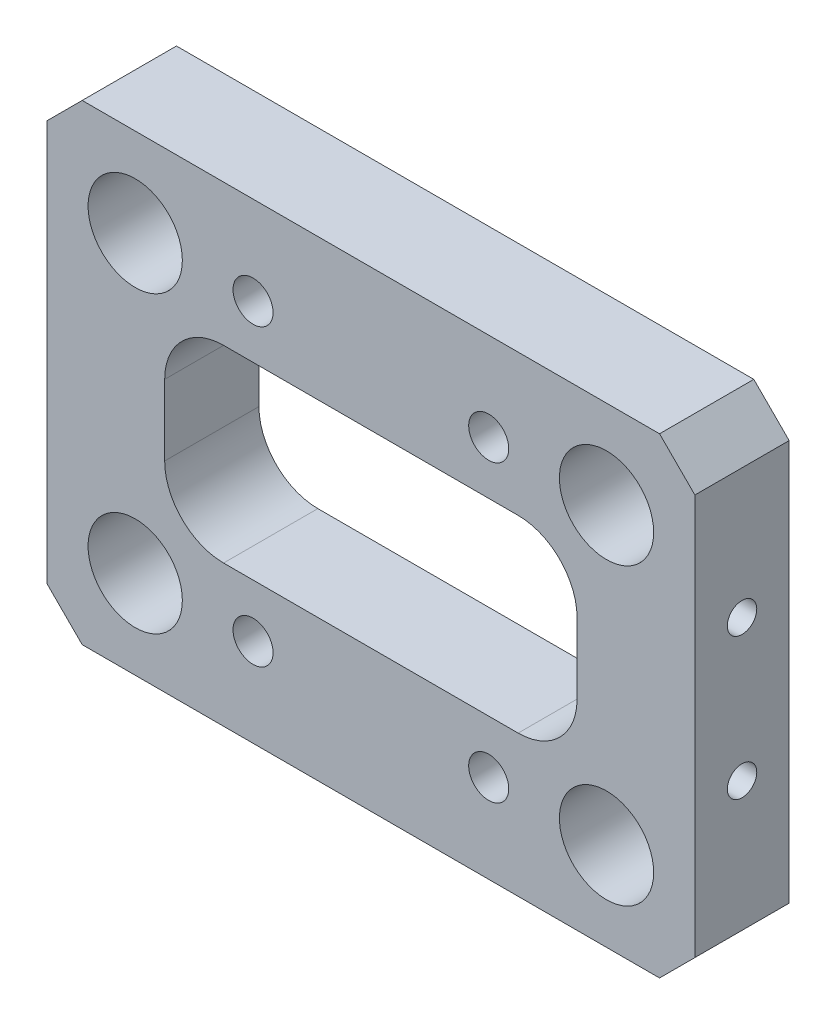
SolidWorks part; units mm, degrees
material "6061-T6 (SS)"
ref_plane "Front" through (0, 0, 0) normal (0, 0, 1) x (1, 0, 0)
ref_plane "Top" through (0, 0, 0) normal (0, 1, 0) x (1, 0, 0)
ref_plane "Right" through (0, 0, 0) normal (1, 0, 0) x (0, 0, -1)
ref_plane "基准面1" through (0, 0, 4) normal (0, 0, 1) x (1, 0, 0)
sketch "草图1" plane through (0, 0, 4) normal (0, 0, 1) x (1, 0, 0)
  line L0 (-27.5, 20) -> (-27.5, -20)
  line L1 (-27.5, -20) -> (27.5, -20)
  line L2 (27.5, -20) -> (27.5, 20)
  line L3 (27.5, 20) -> (-27.5, 20)
  line L4 (0, 0) -> (0, 23.5541) construction
  line L5 (0, 0) -> (-34.4635, 0) construction
  dimension "D1" = 40
  dimension "D2" = 55
extrude "凸台-拉伸1" add sketch "草图1" against normal blind 8
sketch "草图2" plane through (0, 0, -4) normal (0, 0, -1) x (-1, 0, 0)
  line L0 (17.5, -8) -> (17.5, 8)
  line L1 (17.5, 8) -> (-17.5, 8)
  line L2 (-17.5, 8) -> (-17.5, -8)
  line L3 (-17.5, -8) -> (17.5, -8)
  line L4 (0, 0) -> (0, 21.9803) construction
  line L5 (0, 0) -> (35.1489, 0) construction
  dimension "D1" = 35
  dimension "D2" = 16
extrude "切除-拉伸1" cut sketch "草图2" against normal through all
hole_wizard "M3 六角头机械螺钉的柱形沉头孔1" positions "草图4" profile "草图3" counterbore size "M3" standard "ANSI Metric"
sketch "草图4" plane through (0, 0, -4) normal (0, 0, -1) x (-1, 0, 0)
  line L0 (0, 0) -> (0, 22.8615) construction
  line L3 (0, 0) -> (-32.4075, 0) construction
  point P0 (10, -12.5)
  point P1 (-10, -12.5)
  point P2 (10, 12.5)
  point P3 (-10, 12.5)
  dimension "D1" = 20
  dimension "D2" = 25
sketch "草图3" plane through (-10, -12.5, -4) normal (1, 0, 0) x (0, 1, 0)
  line L0 (0, 0) -> (0, 8)
  line L1 (0, 8) -> (1.7, 8)
  line L3 (1.7, 8) -> (1.7, 3.4)
  line L4 (1.7, 3.4) -> (3, 3.4)
  line L5 (3, 3.4) -> (3, 0)
  line L7 (3, 0) -> (0, 0)
  line L11 (0, -6.35) -> (0, 107.95) construction
  dimension "通孔孔直径" = 3.4
  dimension "通孔孔深度" = 8
  dimension "柱形沉头孔直径" = 6
  dimension "柱形沉头孔深度" = 3.4
hole_wizard "M3 螺纹孔1" positions "草图6" profile "草图5" tap size "M3" standard "GB"
sketch "草图6" plane through (27.5, 0, 0) normal (1, 0, 0) x (0, 0, -1)
  line L0 (0, 0) -> (-6.2677, 0) construction
  line L3 (0, 0) -> (0, 23.4526) construction
  point P0 (0, 6)
  point P1 (0, -6)
  dimension "D1" = 12
sketch "草图5" plane through (27.5, 6, 0) normal (0, 1, 0) x (0, 0, -1)
  line L0 (0, 0) -> (0, 8.2511)
  line L1 (0, 8.2511) -> (1.25, 7.5)
  line L2 (1.25, 7.5) -> (1.25, 0)
  line L5 (1.25, 0) -> (0, 0)
  line L10 (0, 8.2511) -> (-1.25, 7.5) construction
  line L11 (0, -6.35) -> (0, 107.95) construction
  dimension "螺纹孔钻头直径" = 2.5
  dimension "螺纹孔钻头深度" = 7.5
  dimension "导头角度" = 118
cosmetic thread "孔螺蚊线1" parameters "D1"=6, "D2"=3
cosmetic thread "孔螺蚊线2" parameters "D1"=6, "D2"=3
hole_wizard "M8x1.0 螺纹孔1" positions "草图8" profile "草图7" tap size "M8x1.0" standard "ANSI Metric" end condition through all
sketch "草图8" plane through (0, 0, 4) normal (0, 0, 1) x (1, 0, 0)
  line L0 (0, 0) -> (-30.9361, 0) construction
  line L3 (0, 0) -> (0, 21.9885) construction
  point P0 (-20, 12.5)
  point P1 (-20, -12.5)
  point P2 (20, 12.5)
  point P3 (20, -12.5)
  dimension "D1" = 40
  dimension "D2" = 25
sketch "草图7" plane through (-20, 12.5, 4) normal (1, 0, 0) x (0, -1, 0)
  line L0 (0, 0) -> (0, 8)
  line L1 (0, 8) -> (2.5, 8)
  line L3 (2.5, 8) -> (2.5, 6)
  line L4 (2.5, 6) -> (4, 6)
  line L5 (4, 6) -> (4, 0)
  line L7 (4, 0) -> (0, 0)
  line L11 (0, -6.35) -> (0, 107.95) construction
  dimension "通孔螺纹孔钻头直径" = 5
  dimension "通孔螺纹孔钻头深度" = 8
  dimension "螺纹线主直径" = 8
  dimension "螺纹线深度" = 6
hole_wizard "M3 螺纹孔2" positions "草图10" profile "草图9" tap size "M3" standard "GB"
sketch "草图10" plane through (-27.5, 0, 0) normal (-1, 0, 0) x (0, 0, 1)
  line L0 (0, 0) -> (7.8326, 0) construction
  line L3 (0, 0) -> (0, 25.2112) construction
  point P0 (0, 6)
  point P1 (0, -6)
  dimension "D1" = 12
sketch "草图9" plane through (-27.5, 6, 0) normal (0, 1, 0) x (0, 0, 1)
  line L0 (0, 0) -> (0, 9.2511)
  line L1 (0, 9.2511) -> (1.25, 8.5)
  line L2 (1.25, 8.5) -> (1.25, 0)
  line L5 (1.25, 0) -> (0, 0)
  line L10 (0, 9.2511) -> (-1.25, 8.5) construction
  line L11 (0, -6.35) -> (0, 107.95) construction
  dimension "螺纹孔钻头直径" = 2.5
  dimension "螺纹孔钻头深度" = 8.5
  dimension "导头角度" = 118
cosmetic thread "孔螺蚊线3" parameters "D1"=6, "D2"=3
cosmetic thread "孔螺蚊线4" parameters "D1"=6, "D2"=3
chamfer "倒角1" distance 3 angle 45 4 edges at (-27.5, 20, 0) (-27.5, -20, 0) (27.5, 20, 0) (27.5, -20, 0)
fillet "圆角1" radius 5 4 edges at (-17.5, -8, 0) (17.5, -8, 0) (-17.5, 8, 0) (17.5, 8, 0)
